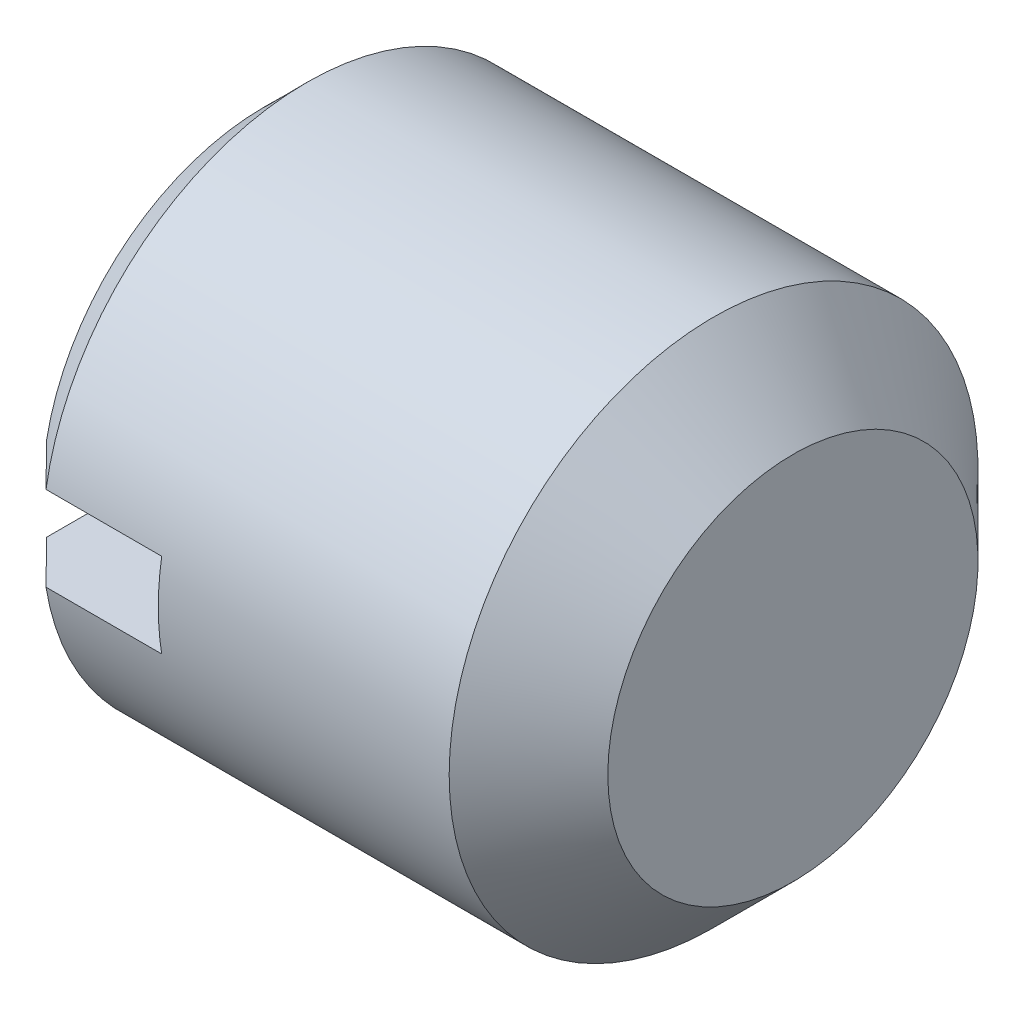
from build123d import *

# Parameters (mm, degrees)
NOTCH_DEPTH      = 13.247448714
NOTCH_DEPTH_BACK = 13.247448714
SKETCH2_W        = 3
SKETCH2_H        = 1.6


with BuildPart() as part:
    # Sketch1 → Base (revolve)
    with BuildSketch(Plane.XY, mode=Mode.PRIVATE) as base_sk:
        Polygon((0, 0), (10, 0), (10, 3.5), (8.5, 5), (0.812, 5), (0, 4.188), align=None)
    revolve(base_sk.sketch.rotate(Axis((-10.745014543, 0, 0), (1, 0, 0)), 90), axis=Axis((-10.745014543, 0, 0), (1, 0, 0)))

    # Sketch2 → Notch (cut, two sides: drawn at the far end of the back side and taken through both)
    with BuildSketch(Plane.XY.offset(-NOTCH_DEPTH_BACK)):
        with Locations((1.5, 0)):
            Rectangle(SKETCH2_W, SKETCH2_H)
    extrude(amount=NOTCH_DEPTH + NOTCH_DEPTH_BACK, mode=Mode.SUBTRACT)


solid = part.part
